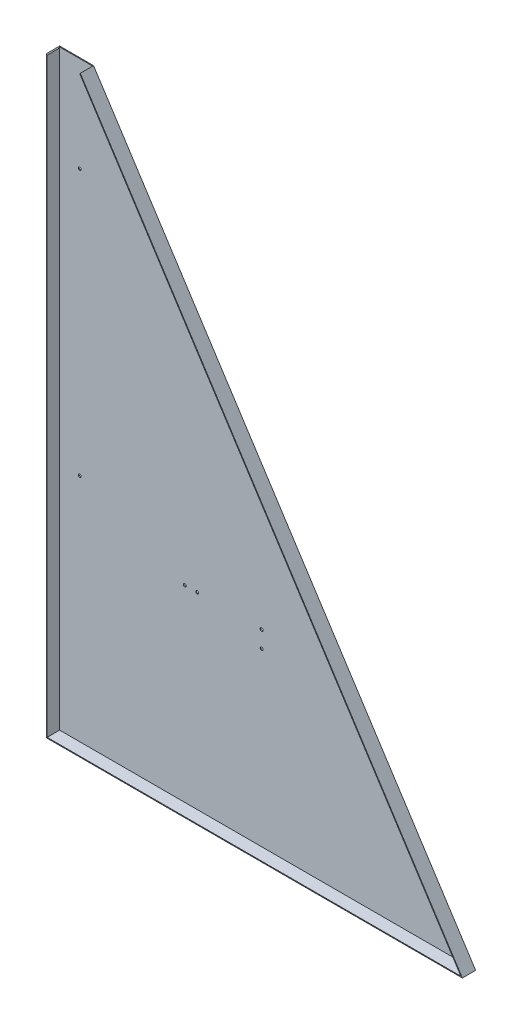
SolidWorks part; units mm, degrees
material "1023 碳钢板 (SS)"
ref_plane "Front Plane" through (0, 0, 0) normal (0, 0, 1) x (1, 0, 0)
ref_plane "Top Plane" through (0, 0, 0) normal (0, 1, 0) x (1, 0, 0)
ref_plane "Right Plane" through (0, 0, 0) normal (1, 0, 0) x (0, 0, -1)
sketch "Sketch1" plane through (0, 0, 0) normal (0, 0, 1) x (1, 0, 0)
  line L1 (-501, 713.5) -> (501, 713.5)
  line L2 (-501, 713.5) -> (-501, -713.5)
  line L3 (-501, -713.5) -> (501, -713.5)
  line L4 (501, 713.5) -> (501, -713.5)
  line L5 (-501, 713.5) -> (501, -713.5) construction
  line L6 (-501, -713.5) -> (501, 713.5) construction
  point P0 (0, 0)
  dimension "D1" = 1002
  dimension "D2" = 1427
extrude "Boss-Extrude1" add sketch "Sketch1" along normal blind 2
sketch "Sketch2" plane through (0, 0, 2) normal (0, 0, 1) x (1, 0, 0)
  line L0 (-419.25, 713.5) -> (501, -713.5)
  line L2 (501, -713.5) -> (501, 713.5) construction
  line L3 (-419.25, 713.5) -> (501, 713.5)
  line L4 (501, 713.5) -> (501, -713.5)
  line L5 (-501, -713.5) -> (501, -713.5) construction
  dimension "D1" = 1427
  dimension "D2" = 920.25
extrude "Cut-Extrude1" cut sketch "Sketch2" against normal blind 2
sketch "Sketch5" plane through (0, 0, 2) normal (0, 0, 1) x (1, 0, 0)
  line L0 (-501, 713.5) -> (-501, -713.5) construction
  line L1 (-501, -713.5) -> (501, -713.5) construction
  circle A0 centre (-197.5, -258.5) radius 3.5
  circle A1 centre (-167.5, -258.5) radius 3.5
  circle A2 centre (-12.5, -258.5) radius 3.5
  circle A3 centre (-12.5, -298.5) radius 3.5
  dimension "D3" = 303.5
  dimension "D6" = 7
  dimension "D1" = 30
  dimension "D2" = 40
  dimension "D4" = 155
  dimension "D5" = 455
extrude "Cut-Extrude2" cut sketch "Sketch5" against normal blind 40
sketch "Sketch6" plane through (0, 0, 2) normal (0, 0, 1) x (1, 0, 0)
  line L0 (-499, 711.5) -> (-499, -711.5)
  line L1 (-499, -711.5) -> (497.3304, -711.5)
  line L2 (497.3304, -711.5) -> (-420.34, 711.5)
  line L4 (501, -713.5) -> (-419.25, 713.5)
  line L5 (-419.25, 713.5) -> (-501, 713.5)
  line L6 (-501, 713.5) -> (-501, -713.5)
  line L7 (-501, -713.5) -> (501, -713.5)
  line L8 (501, -713.5) -> (-419.25, 713.5)
  line L10 (-501, 713.5) -> (-501, -713.5)
  line L11 (-501, -713.5) -> (501, -713.5)
  line L12 (-420.34, 711.5) -> (-499, 711.5) construction
  line L13 (-419.25, 713.5) -> (-501, 713.5) construction
  line L18 (-499, 711.5) -> (-501, 713.5)
  line L19 (-419.25, 713.5) -> (-420.34, 711.5)
  dimension "D1" = 0
  dimension "D2" = 2
extrude "Boss-Extrude2" add sketch "Sketch6" along normal blind 30
sketch "Sketch7" plane through (0, 0, 2) normal (0, 0, 1) x (1, 0, 0)
  line L0 (-419.25, 713.5) -> (-501, 713.5) construction
  line L1 (-499, -711.5) -> (-499, 711.5) construction
  circle A0 centre (-450.5, 483.5) radius 3.5
  circle A1 centre (-450.5, -156.5) radius 3.5
  dimension "D4" = 7
  dimension "D5" = 7
  dimension "D1" = 640
  dimension "D2" = 230
  dimension "D3" = 48.5
extrude "Cut-Extrude3" cut sketch "Sketch7" against normal blind 10
